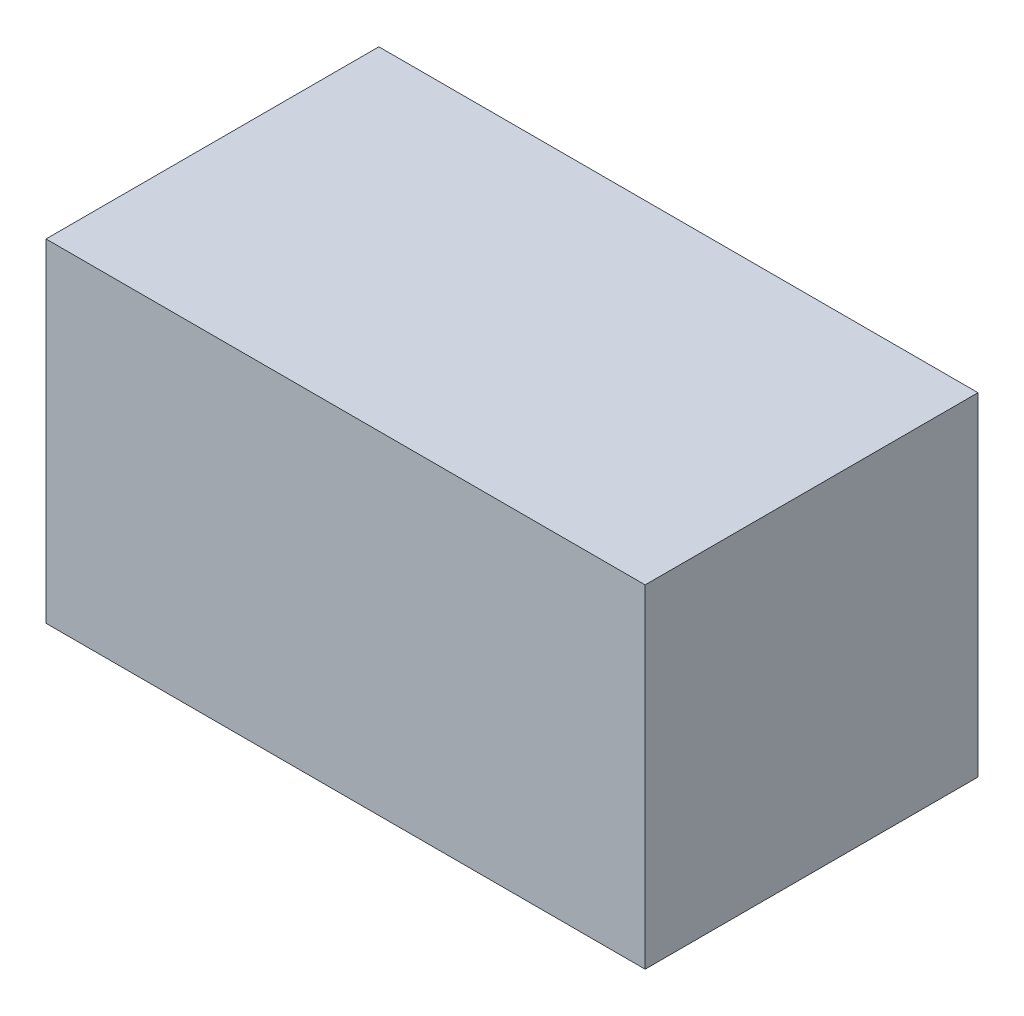
SolidWorks part; units mm, degrees
ref_plane "前视基准面" through (0, 0, 0) normal (0, 0, 1) x (1, 0, 0)
ref_plane "上视基准面" through (0, 0, 0) normal (0, 1, 0) x (1, 0, 0)
ref_plane "右视基准面" through (0, 0, 0) normal (1, 0, 0) x (0, 0, -1)
other "Configuration Table"
sketch "草图1" plane through (0, 0, 0) normal (0, 0, 1) x (1, 0, 0)
  line L0 (-9, -5) -> (9, -5)
  line L1 (9, -5) -> (9, 5)
  line L2 (9, 5) -> (-9, 5)
  line L3 (-9, 5) -> (-9, -5)
  point P0 (0, 0)
  dimension "D1" = 9
  dimension "D2" = 18
  dimension "D3" = 5
  dimension "D4" = 10
extrude "凸台-拉伸1" add sketch "草图1" against normal mid plane 10
